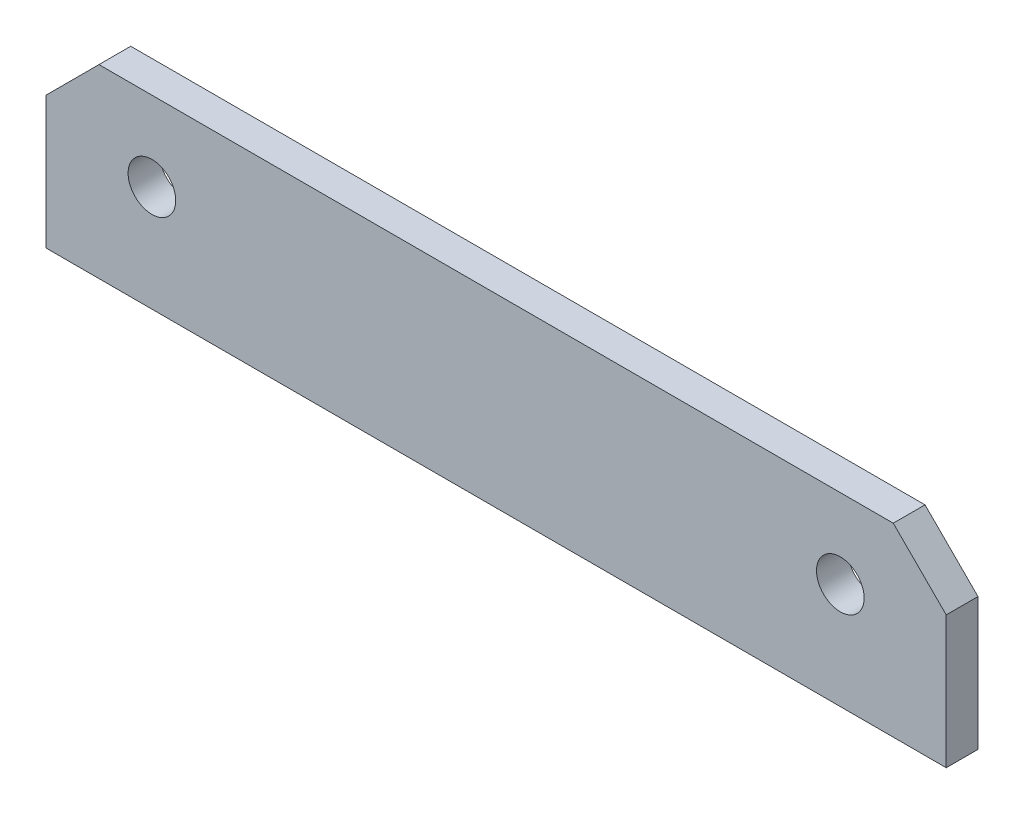
from build123d import *

# Parameters (mm, degrees)
BOSS_EXTRUDE1_DEPTH = 1.5
SKETCH2_R           = 2.25
CUT_EXTRUDE1_DEPTH  = 3


with BuildPart() as part:
    # Sketch1 → Boss-Extrude1 (new, symmetric)
    with BuildSketch(Plane.XY):
        Polygon((-646.5, 109.2), (-561.5, 109.2), (-561.5, 121.7), (-566.5, 126.7), (-641.5, 126.7), (-646.5, 121.7), align=None)
    extrude(amount=BOSS_EXTRUDE1_DEPTH, both=True)

    # Sketch2 → Cut-Extrude1 (cut)
    with BuildSketch(Plane.XY.offset(1.5)):
        with Locations((-636.5, 119.2)):
            Circle(SKETCH2_R)
        with Locations((-571.5, 119.2)):
            Circle(SKETCH2_R)
    extrude(amount=-CUT_EXTRUDE1_DEPTH, mode=Mode.SUBTRACT)


solid = part.part
